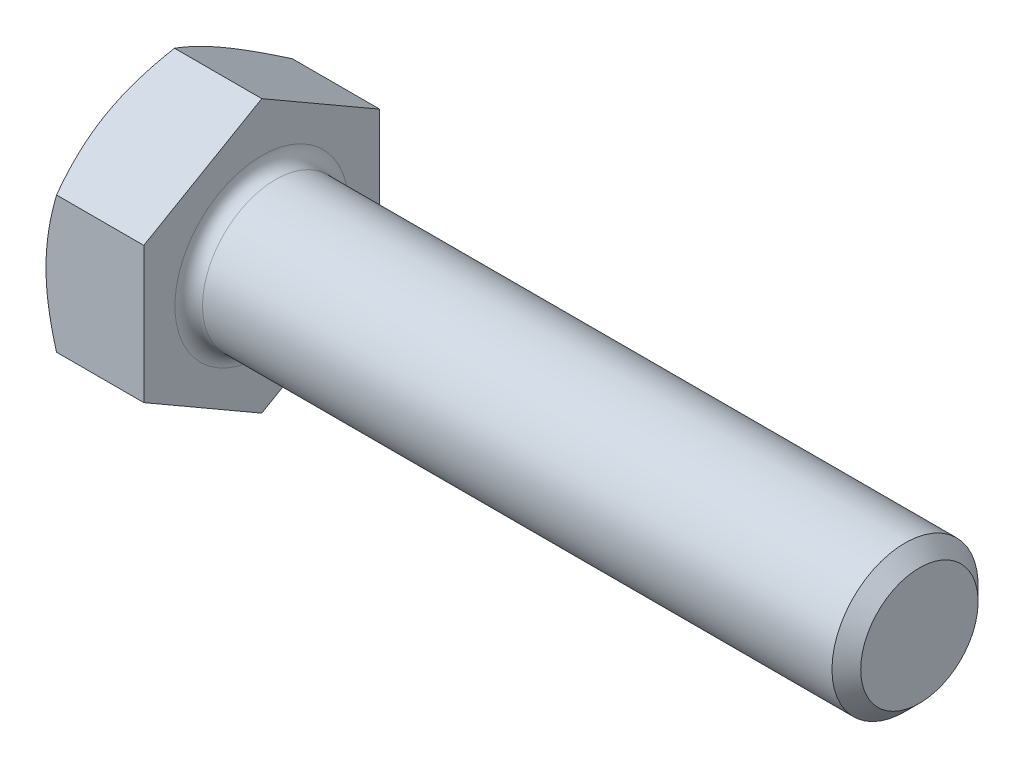
SolidWorks part; units mm, degrees
material "SAE5"
ref_plane "Front plane" through (0, 0, 0) normal (0, 0, 1) x (1, 0, 0)
ref_plane "Top plane" through (0, 0, 0) normal (0, 1, 0) x (1, 0, 0)
ref_plane "Right plane" through (0, 0, 0) normal (1, 0, 0) x (0, 0, -1)
sketch "Sketch1" plane through (0, 0, 0) normal (1, 0, 0) x (0, 0, -1)
  line L0 (20.5, 11.8357) -> (20.5, -11.8357)
  line L1 (-20.5, 11.8357) -> (-20.5, -11.8357)
  line L2 (20.5, -11.8357) -> (0, -23.6714)
  line L3 (0, -23.6714) -> (-20.5, -11.8357)
  line L4 (20.5, 11.8357) -> (0, 23.6714)
  line L5 (0, 23.6714) -> (-20.5, 11.8357)
  dimension "s" = 41
  dimension "D2" = 120
  dimension "D3" = 20.5
  dimension "D4" = 20.5
  dimension "D5" = 20.5
extrude "Base-Extrude" add sketch "Sketch1" along normal blind 17
sketch "Sketch2" plane through (0, 0, 0) normal (0, 0, 1) x (1, 0, 0)
  line L0 (0, 11.8357) -> (0, -11.8357) construction
  line L1 (0, 0) -> (131.3, 0)
  line L2 (0, 0) -> (0, 12.7)
  line L3 (0, 12.7) -> (27.8072, 12.7)
  line L4 (131.3, 0) -> (131.3, 10.902)
  line L5 (17, 23.6714) -> (17, 11.8357) construction
  line L7 (0, 0) -> (96.52, 0) construction
  line L8 (131.3, -10.902) -> (27.8072, -12.7) construction
  line L9 (0, -12.7) -> (27.8072, -12.7) construction
  line L10 (20, 15.24) -> (20, -1.27) construction
  line L11 (74.15, 15.24) -> (74.15, -1.27) construction
  line L12 (17, 11.8357) -> (17, -11.8357) construction
  line L13 (27.8072, 12.7) -> (131.3, 12.7)
  line L14 (131.3, 12.7) -> (131.3, 10.902)
  dimension "l" = 114.3
  dimension "m" = 25.4
  dimension "Minor_dia" = 21.804
  dimension "p" = 3
  dimension "h" = 57.15
revolve "Boss-Revolve1" add sketch "Sketch2" angle 360 about L7
cosmetic thread "Helix1" parameters "Thread_length"=60, "Thread_minor"=21.804
sketch "Sketch3" plane through (0, 0, 0) normal (0, 0, 1) x (1, 0, 0)
  line L0 (0, 20.5) -> (4.7177, 28.6714)
  line L1 (0, 23.6714) -> (0, 11.8357) construction
  line L2 (4.7177, 28.6714) -> (4.7177, 33.6714)
  line L3 (4.7177, 33.6714) -> (-10, 33.6714)
  line L4 (-10, 33.6714) -> (-10, 20.5)
  line L5 (-10, 20.5) -> (0, 20.5)
  line L6 (0, 0) -> (99.06, 0) construction
  line L7 (17, 23.6714) -> (0, 23.6714) construction
  dimension "D1" = 20.5
  dimension "D2" = 5
  dimension "D3" = 10
  dimension "D4" = 5
  dimension "Head_ch_ang" = 30
revolve "Cut-Revolve1" cut sketch "Sketch3" angle 360 about L6
sketch "Sketch5" plane through (0, 0, 0) normal (0, 0, 1) x (1, 0, 0)
  line L0 (17, 20.5) -> (12.2823, 28.6714)
  line L1 (17, 23.6714) -> (17, 11.8357) construction
  line L2 (12.2823, 28.6714) -> (12.2823, 33.6714)
  line L3 (12.2823, 33.6714) -> (22.2823, 33.6714)
  line L4 (22.2823, 33.6714) -> (22.2823, 20.5)
  line L5 (22.2823, 20.5) -> (17, 20.5)
  line L7 (17, 23.6714) -> (1.831, 23.6714) construction
  line L8 (0, 0) -> (99.06, 0) construction
  line L9 (0, 0) -> (99.06, 0) construction
  dimension "D1" = 20.5
  dimension "D2" = 5
  dimension "D3" = 10
  dimension "Head_ch_ang" = 30
  dimension "D4" = 5
revolve "Cut-Revolve2" [suppressed] cut sketch "Sketch5" angle 360 about L8
sketch "Sketch4" plane through (0, 0, 0) normal (0, 0, 1) x (1, 0, 0)
  line L1 (17, 23.6714) -> (17, 11.8357) construction
  line L2 (17, 20.5) -> (16.2, 20.5)
  line L3 (17, 20.5) -> (17, 33.6714)
  line L4 (17, 33.6714) -> (16.2, 33.6714)
  line L5 (0, 0) -> (95.25, 0) construction
  line L6 (0, 0) -> (96.52, 0) construction
  line L7 (16.2, 20.5) -> (16.2, 33.6714)
  line L8 (17, 23.6714) -> (1.831, 23.6714) construction
  dimension "D1" = 41
  dimension "D2" = 10
  dimension "c" = 0.8
revolve "Cut-Revolve3" [suppressed] cut sketch "Sketch4" angle 360 about L5
chamfer "Chamfer" distance 2.5 angle 45 1 edges at (131.3, 0, 12.7)
fillet "Fillet" radius 2.4 1 edges at (17, 0, -12.7)
sketch "Sketch6" plane through (0, 0, 0) normal (0, 0, 1) x (1, 0, 0)
  line L0 (117, -10.902) -> (115.5, -13.5)
  line L1 (117, -10.902) -> (118.5, -13.5)
  line L2 (118.5, -13.5) -> (118.5, -16.875)
  line L3 (-3.175, 0) -> (5.1513, 0) construction
  line L5 (118.5, -16.875) -> (115.5, -16.875)
  line L6 (115.5, -16.875) -> (115.5, -13.5)
  dimension "Thread_minor" = 21.804
  dimension "Diameter" = 27
  dimension "Start" = 117
  dimension "SideAngle" = 60
  dimension "VeeAngle" = 60
  dimension "Overcut" = 33.75
revolve "Cut-Revolve4" [suppressed] cut sketch "Sketch6" angle 360 about L3
pattern_linear "LPattern1" [suppressed]
